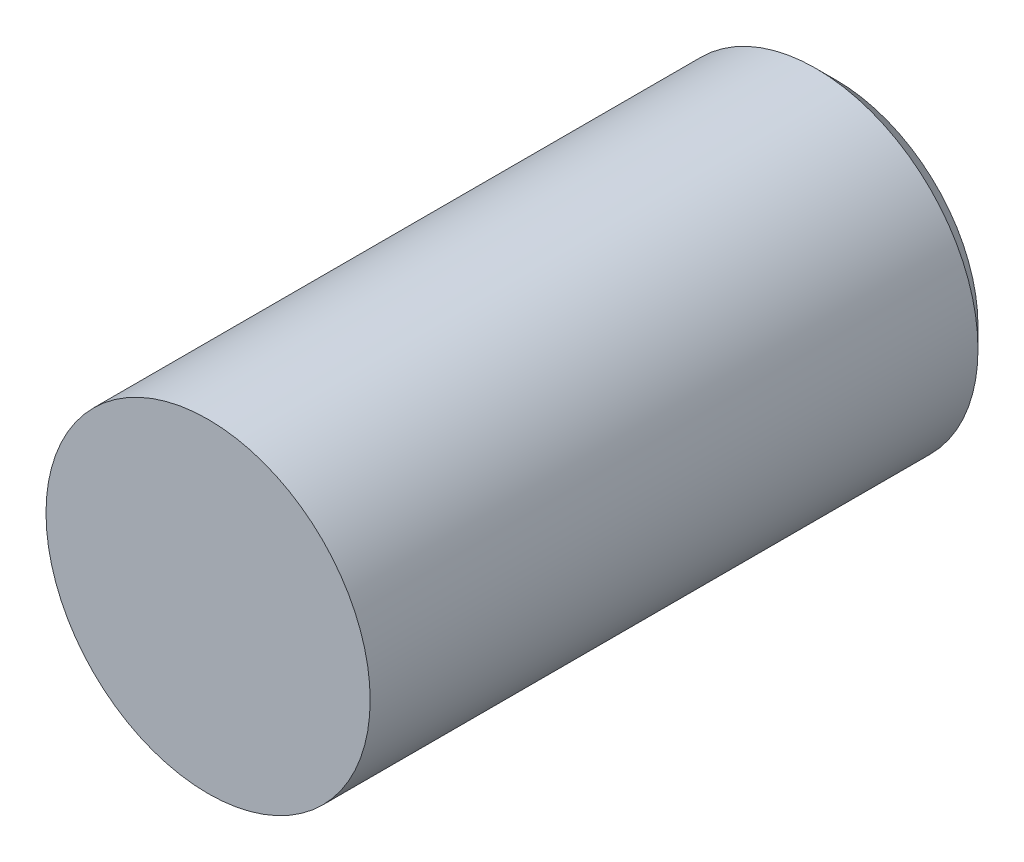
from build123d import *

# Parameters (mm, degrees)
SKETCH1_R           = 8
BOSS_EXTRUDE1_DEPTH = 31
CHAMFER2_SIZE       = 1


with BuildPart() as part:
    # Sketch1 → Boss-Extrude1 (new body)
    with BuildSketch(Plane.XY):
        Circle(SKETCH1_R)
    extrude(amount=BOSS_EXTRUDE1_DEPTH)

    # Chamfer2
    chamfer2_edges = [part.edges().sort_by_distance(p)[0] for p in [
        (-8, 0, 0),
    ]]
    chamfer(chamfer2_edges, length=CHAMFER2_SIZE)


solid = part.part
